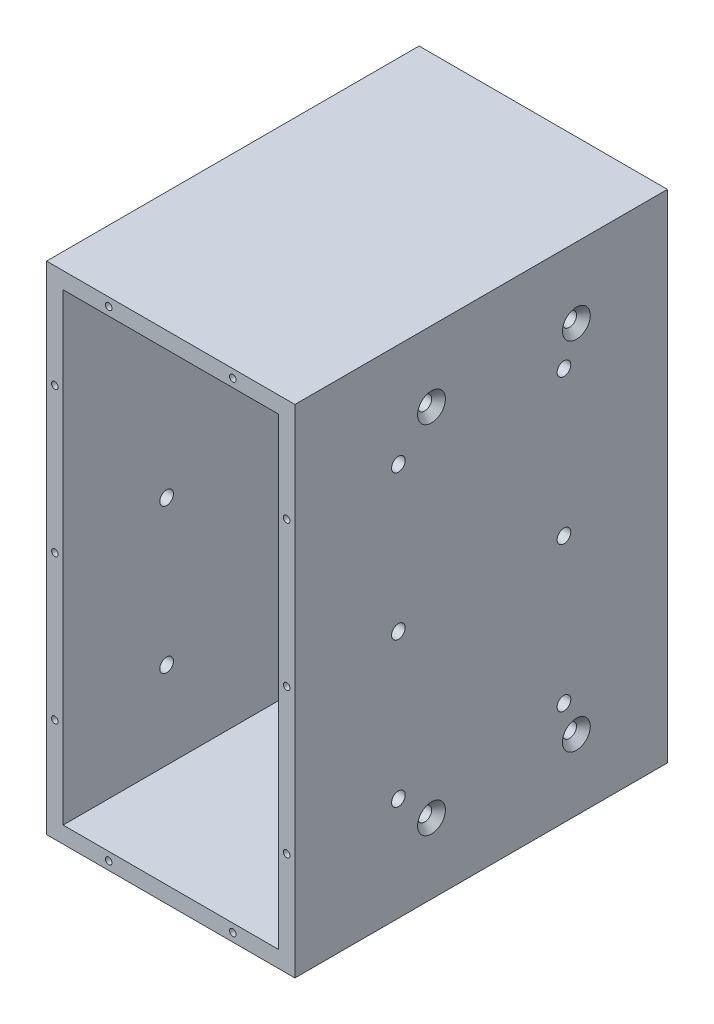
from build123d import *

# Parameters (mm, degrees)
SKETCH_1_W                   = 60
SKETCH_1_H                   = 120
EXTRUDE_1_DEPTH              = 45
SHELL_1_T                    = -4
HOLE_WIZARD_M2_1_D           = 1.6
HOLE_WIZARD_M2_1_DEPTH       = 5.2
HOLE_WIZARD_M2_1_TIP         = 0.480688495
HOLE_WIZARD_M2_2_D           = 1.6
HOLE_WIZARD_M2_2_DEPTH       = 5.2
HOLE_WIZARD_M2_2_TIP         = 0.480688495
HOLE_WIZARD_M3_1_D           = 3.4
HOLE_WIZARD_M3_1_DEPTH       = 4
HOLE_WIZARD_M3_1_CSINK_D     = 6.72
HOLE_WIZARD_M3_1_CSINK_ANGLE = 90
HOLE_WIZARD_M4_1_D           = 3.3


with BuildPart() as part:
    # 草图1 → 凸台-拉伸1 (new, symmetric)
    with BuildSketch(Plane.XY):
        Rectangle(SKETCH_1_W, SKETCH_1_H)
    extrude(amount=EXTRUDE_1_DEPTH, both=True)

    # 抽壳1
    shell_1_openings = [part.faces().sort_by_distance(p)[0] for p in [
        (0, 0, 45),
        (0, 0, -45),
    ]]
    offset(amount=SHELL_1_T, openings=shell_1_openings, kind=Kind.INTERSECTION)

    # M2 螺纹孔1
    with Locations(Plane.XY.offset(45)):
        with Locations((-15, -58), (-28, 0), (28, 0), (-15, 58), (15, 58), (-28, 35), (28, 35), (28, -35), (-28, -35), (15, -58)):
            Hole(HOLE_WIZARD_M2_1_D / 2, depth=HOLE_WIZARD_M2_1_DEPTH)
            with Locations((0, 0, -(HOLE_WIZARD_M2_1_DEPTH + HOLE_WIZARD_M2_1_TIP / 2))):  # 118° drill point
                Cone(0, HOLE_WIZARD_M2_1_D / 2, HOLE_WIZARD_M2_1_TIP, mode=Mode.SUBTRACT)

    # M2 螺纹孔2
    with Locations(Plane(origin=(0, 0, -45), x_dir=(-1, 0, 0), z_dir=(0, 0, -1))):
        with Locations((28, 0), (-28, 0), (-15, 58), (15, 58), (28, 35), (-28, 35), (-28, -35), (28, -35), (-15, -58), (15, -58)):
            Hole(HOLE_WIZARD_M2_2_D / 2, depth=HOLE_WIZARD_M2_2_DEPTH)
            with Locations((0, 0, -(HOLE_WIZARD_M2_2_DEPTH + HOLE_WIZARD_M2_2_TIP / 2))):  # 118° drill point
                Cone(0, HOLE_WIZARD_M2_2_D / 2, HOLE_WIZARD_M2_2_TIP, mode=Mode.SUBTRACT)

    # M3 六角凹锥坑螺钉的锥形沉头孔1
    with Locations(Plane(origin=(30, 0, 0), x_dir=(0, 0, -1), z_dir=(1, 0, 0))):
        with Locations((-12, 43), (23, 43), (-12, -43), (23, -43)):
            CounterSinkHole(HOLE_WIZARD_M3_1_D / 2, HOLE_WIZARD_M3_1_CSINK_D / 2, depth=HOLE_WIZARD_M3_1_DEPTH, counter_sink_angle=HOLE_WIZARD_M3_1_CSINK_ANGLE)

    # M4 螺纹孔1 (through all)
    with Locations(Plane(origin=(30, 0, 0), x_dir=(0, 0, -1), z_dir=(1, 0, 0))):
        with Locations((20, 35), (-20, -35), (-20, 35), (20, -35), (-20, 0), (20, 0)):
            Hole(HOLE_WIZARD_M4_1_D / 2)


solid = part.part
